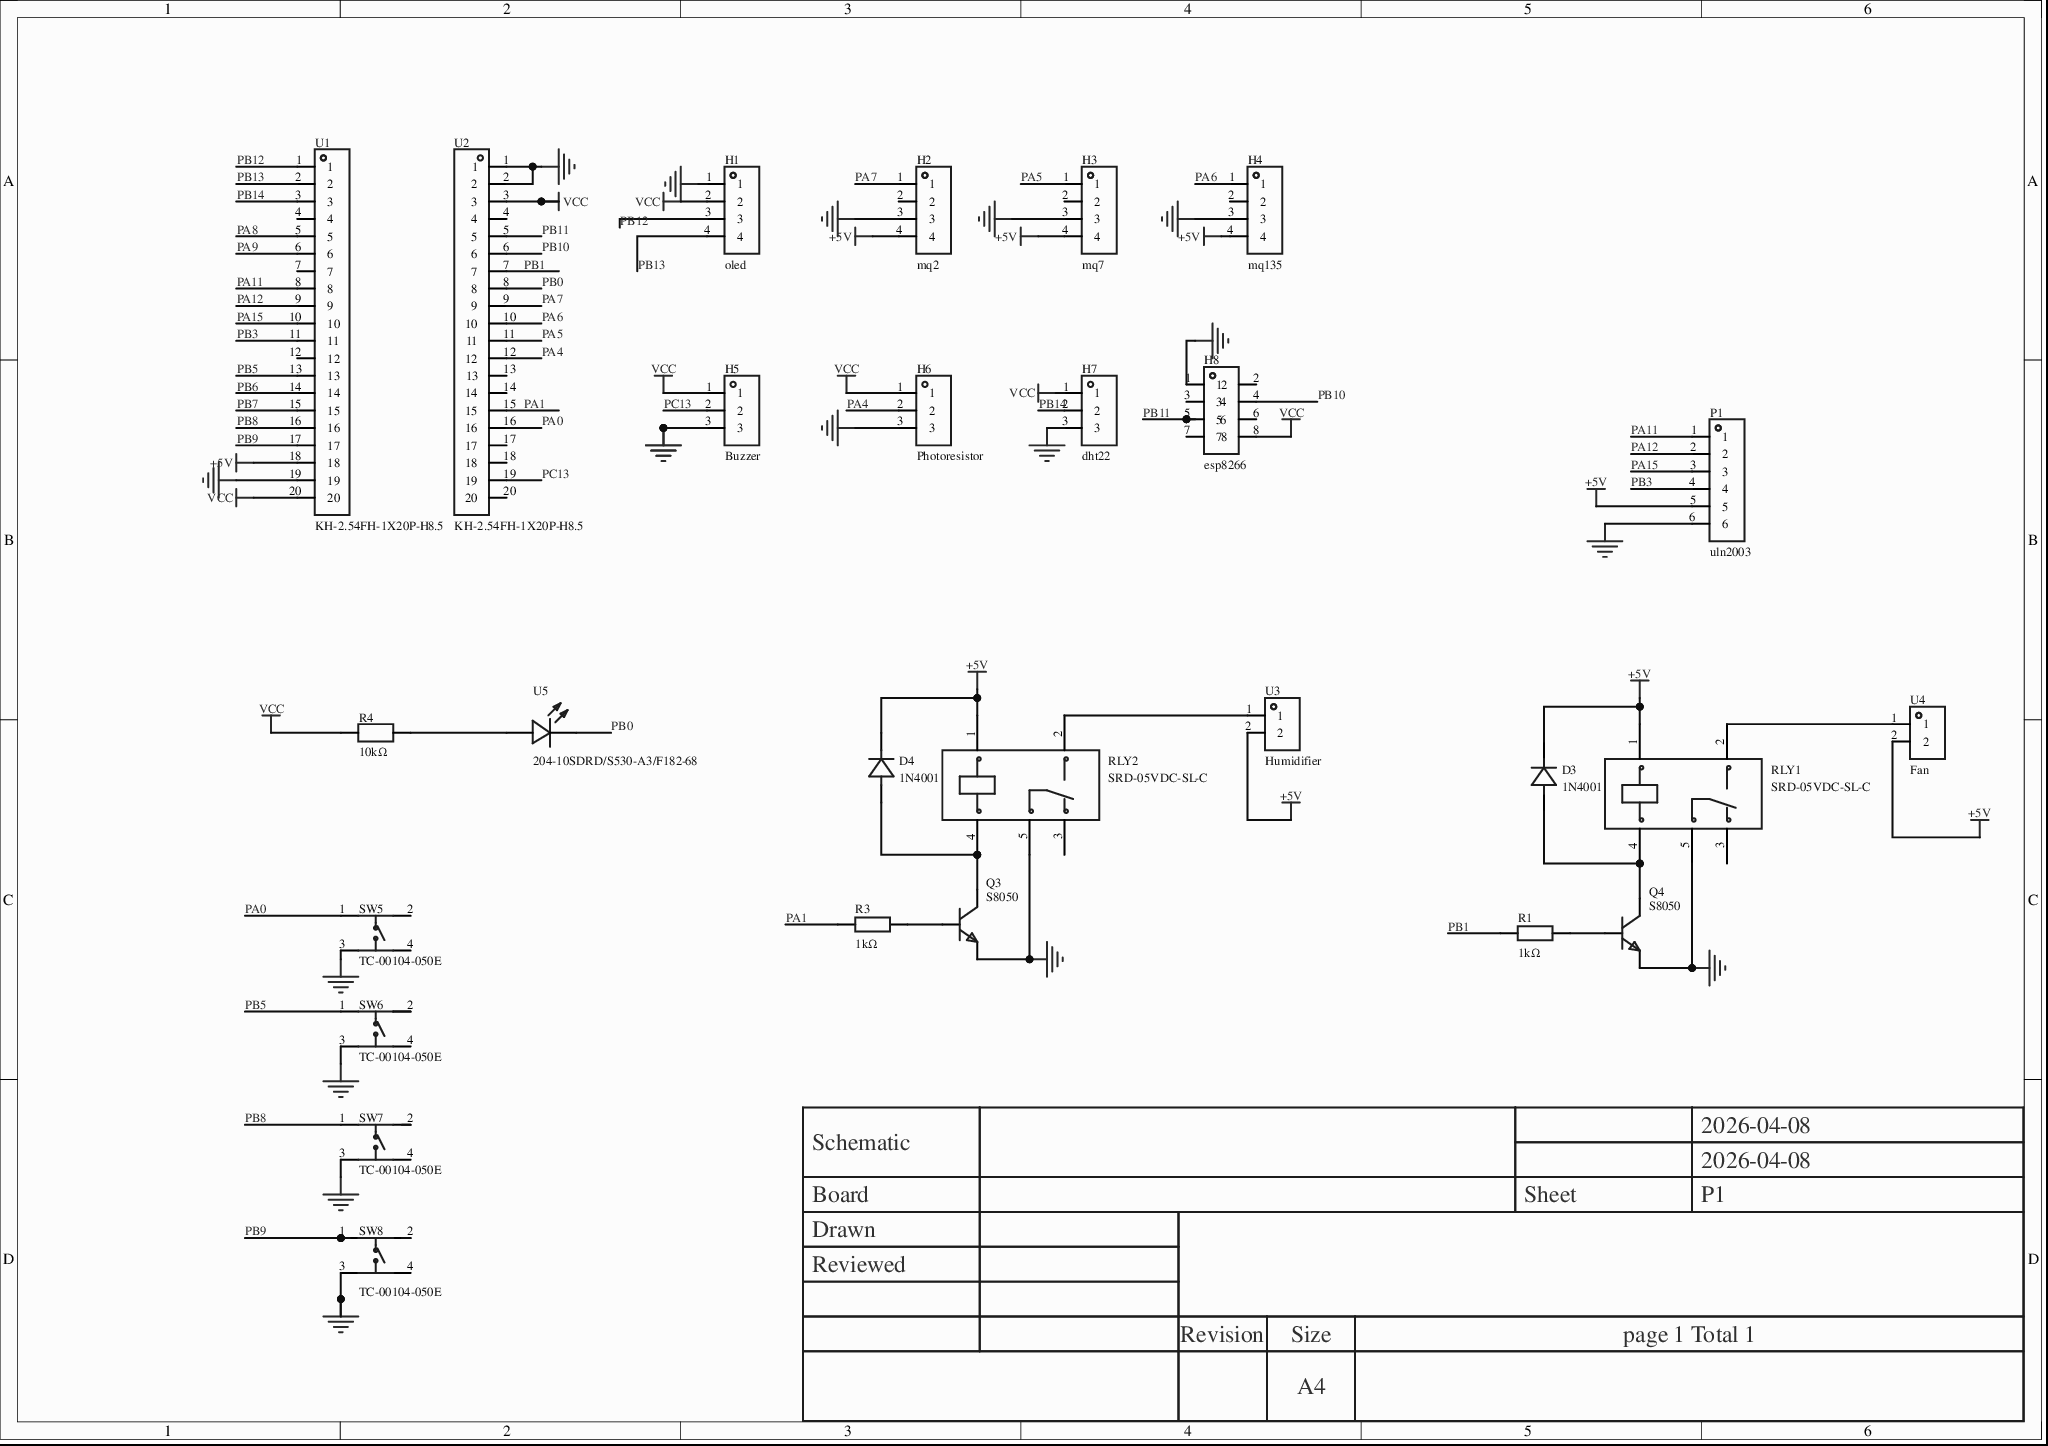
[diagram p0: MISC51563-3.schdoc]
# Altium project MISC51563-2.PrjPcb
1 sheet, 27 parts. Net scope: global (net labels, ports and power ports of the same name join across sheets).
Board file: MISC51563.pcbdoc

## Sheet MISC51563-3.schdoc
size 297 x 209 mm; Version: V1.0; @Project Name: MISC51563; @Update Date: 2026-04-22; @Create Date: 2026-04-22; @Board Name: MISC51563; @Create Time: 22:07:17; @Page Count: 1; @Page No: 1; @Schematic Name: MISC51563; @Update Time: 22:07:17; Size: A4

### Parts
D3  1N4001  [DO-41_BD2.4-L4.7-P8.70-D0.9-RD]
D4  1N4001  [DO-41_BD2.4-L4.7-P8.70-D0.9-RD]
H1  oled  [HDR-TH_4P-P2.54-V-F]
H2  mq2  [HDR-TH_4P-P2.54-V-F]
H3  mq7  [HDR-TH_4P-P2.54-V-F]
H4  mq135  [HDR-TH_4P-P2.54-V-F]
H5  Buzzer  [HDR-TH_3P-P2.54-V-F]
H6  Photoresistor  [HDR-TH_3P-P2.54-V-F]
H7  dht22  [HDR-TH_3P-P2.54-V-F]
H8  esp8266  [HDR-TH_8P-P2.54-V-F-R2-C4-S2.54]
P1  uln2003  [HDR-TH_6P-P2.54-V-F]
Q3  S8050  [TO-92-3_L4.5-W3.5-P1.27-L]
Q4  S8050  [TO-92-3_L4.5-W3.5-P1.27-L]
R1  1kΩ  [RES-TH_BD2.5-L6.5-P10.50-D0.6]
R3  1kΩ  [RES-TH_BD2.5-L6.5-P10.50-D0.6]
R4  10kΩ  [RES-TH_BD2.7-L6.2-P10.20-D0.4]
RLY1  SRD-05VDC-SL-C  [RELAY-TH_SRD-XXVDC-XL-C]
RLY2  SRD-05VDC-SL-C  [RELAY-TH_SRD-XXVDC-XL-C]
SW5  TC-00104-050E  [SW-TH_4P-L6.0-W6.0-P4.50-LS6.5]
SW6  TC-00104-050E  [SW-TH_4P-L6.0-W6.0-P4.50-LS6.5]
SW7  TC-00104-050E  [SW-TH_4P-L6.0-W6.0-P4.50-LS6.5]
SW8  TC-00104-050E  [SW-TH_4P-L6.0-W6.0-P4.50-LS6.5]
U1  KH-2.54FH-1X20P-H8.5  [HDR-TH_20P-P2.54-V-F-2]
U2  KH-2.54FH-1X20P-H8.5  [HDR-TH_20P-P2.54-V-F-2]
U3  Humidifier  [HDR-TH_2P-P2.54-V-F]
U4  Fan  [HDR-TH_2P-P2.54-V-F]
U5  204-10SDRD/S530-A3/F182-68  [LED-TH_BD4.0-P2.50-RD]

### Nets
+5V: D3.1(K) D4.1(K) H2.4 H3.4 H4.4 P1.5 RLY1.1 RLY2.1 U1.18 U3.2 U4.2
GND: H1.1 H2.3 H3.3 H4.3 H5.3 H6.3 H7.3 H8.1 P1.6 Q3.1(E) Q4.1(E) RLY1.5 RLY2.5 SW5.3(C) SW6.3(C) SW7.3(C) SW8.3(C) U1.19 U2.1 U2.2
VCC: H1.2 H5.1 H6.1 H7.1 H8.8 R4.1 U1.20 U2.3
PA0: SW5.1(A) U2.16
PA1: R3.1 U2.15
PA4: H6.2 U2.12
PA5: H3.1 U2.11
PA6: H4.1 U2.10
PA7: H2.1 U2.9
PA8: U1.5
PA9: U1.6
PA11: P1.1 U1.8
PA12: P1.2 U1.9
PA15: P1.3 U1.10
PB0: U2.8 U5.1(C)
PB1: R1.1 U2.7
PB3: P1.4 U1.11
PB5: SW6.1(A) U1.13
PB6: U1.14
PB7: U1.15
PB8: SW7.1(A) U1.16
PB9: SW8.1(A) U1.17
PB10: H8.4 U2.6
PB11: H8.5 U2.5
PB12: H1.3 U1.1
PB13: H1.4 U1.2
PB14: H7.2 U1.3
PC13: H5.2 U2.19
NetD3_2: D3.2(A) Q4.3(C) RLY1.4
NetD4_2: D4.2(A) Q3.3(C) RLY2.4
NetQ3_2: Q3.2(B) R3.2
NetQ4_2: Q4.2(B) R1.2
NetR4_2: R4.2 U5.2(A)
NetRLY1_2: RLY1.2 U4.1
NetRLY2_2: RLY2.2 U3.1

Not connected (* = marked no-connect by the designer): H2 2; H3 2; H4 2; H8 2 3 6 7; RLY1 3; RLY2 3; SW5 2(B) 4(D); SW6 2(B) 4(D); SW7 2(B) 4(D); SW8 2(B) 4(D); U1 4 7 12; U2 4 13 14 17 18 20

### Notes on the sheet
- 2026-04-08
- Schematic
- Board
- Sheet
- P1
- Drawn
- Reviewed
- Revision
- Size
- A4
- page 1 Total 1

### Library data of the parts
D3 D4 = 1N4001_C5359862: Diode configuration: independent; forward voltage drop (Vf): 1V@1A; DC reverse withstand voltage (Vr): 50V; rectified current: 1A;; Manufacturer: LGE(鲁光); AddInBom: yes; Reverse Leakage Current (Ir): 5uA@50V; Operating Junction Temperature Range: -65℃~+150℃; ModelId: 6de1e9b71a0d4751b4e9df530304c1a30819f05c4eef4c71ace90d822a990e87; ModelName: DO-41_D2.4-L4.7-P8.70; ModelTransform: 373.9,94.4,232.29,0,0,0,0,0,-140; Device: 1N4001_C5359862; Symbol: 1N4001_C5359862; FootprintName: DO-41_BD2.4-L4.7-P8.70-D0.9-RD; LCSC Part Name: 50V 1A; SupplierPart: C5359862; ManufacturerPart: 1N4001; Supplier Footprint: DO-41; JLCPCB Part Class: Extended Part; Datasheet: example.com/datasheet/1N4001/6175385.html; Supplier: LCSC; ConvertToPcb: yes; Diode Configuration: Independent; Voltage - Forward(Vf@If): 1V@1A; Voltage - DC Reverse(Vr): 50V; Current - Rectified: 1A; Non-Repetitive Peak Forward Surge Current: -
H1-H4 = 2.54-1*4P母: Socket structure: 1x4P; pitch: 2.54mm; row spacing: -; round/square hole: square hole; mounting: through-hole; rows: single row; total positions: 4P; rated current: 3A; rated voltage: -; hole direction: top; plastic height: -; contact material: bronze; contact plating: -; operating temperature: -40℃~+105℃;; Manufacturer: BOOMELE(博穆精密); Device: 2.54-1*4P female; AddInBom: yes; ModelId: d187812051054f85879fcaa51a310d8e0819f05c4eef4c71ace90d822a990e87; ModelTransform: 419.6842,98.464,0,0,0,0,0,0,-118.11; Symbol: 2.54-1*4P female; FootprintName: HDR-TH_4P-P2.54-V-F; LCSC Part Name: 间距:2.54mm 1x4P 直插; SupplierPart: C2718488; Supplier Footprint: 插件,P=2.54mm; JLCPCB Part Class: Extended Part; Datasheet: example.com/datasheet/2.54-1*4P%25E6%25AF%258D/2834502.html; Supplier: LCSC; ConvertToPcb: yes; Holes Structure: 1x4P; Pitch: 2.54mm; Row Spacing: -; Circular Hole / Square Hole: Square hole; Mounting Type: Through-hole; Number of Rows: Single row; Number of Positions: 4P; Current Rating: 3A; Voltage Rating (Max): -; Holes Direction: Top; Insulation Height: -; Contact Material: Bronze; Contact Plating: -; Operating Temperature: -40℃~+105℃; ModelName: HDR-TH_4P-P2.54-V-F
  H1: Manufacturer Part: oled
  H2: Manufacturer Part: mq2
  H3: Manufacturer Part: mq7
  H4: Manufacturer Part: mq135
H5 = PM254V-11-03-H85: Socket structure: 1x3P; pitch: 2.54mm; row spacing: -; round/square hole: square hole; mounting: through-hole; rows: single row; total positions: 3P; rated current: 3A; hole direction: top; plastic height: 8.5mm; contact material: brass; contact plating: -; operating temperature: -40℃~+105℃;; Manufacturer Part: 蜂鸣器; Manufacturer: XFCN(兴飞); AddInBom: yes; ModelId: f3b3cc5aae9641bf9e56fc160cef875b0819f05c4eef4c71ace90d822a990e87; ModelName: HDR2.54-F-LI-1X3P; ModelTransform: 299.9994,100,0,0,0,0,0,0,-118.11; Device: PM254V-11-03-H85; Symbol: PM254V-11-03-H85; FootprintName: HDR-TH_3P-P2.54-V-F; LCSC Part Name: 1x3P 间距:2.54mm 直插; SupplierPart: C541850; Supplier Footprint: 插件,P=2.54mm; JLCPCB Part Class: Extended Part; Datasheet: example.com/datasheet/PM254V-11-03-H85/562471.html; Supplier: LCSC; ConvertToPcb: yes; Holes Structure: 1x3P; Pitch: 2.54mm; Row Spacing: -; Circular Hole / Square Hole: Square hole; Mounting Type: Through-hole; Number of Rows: Single row; Number of Positions: 3P; Current Rating: 3A; Holes Direction: Top; Insulation Height: 8.5mm; Contact Material: Brass; Contact Plating: -; Operating Temperature: -40℃~+105℃
H6 = PM254V-11-03-H85: Socket structure: 1x3P; pitch: 2.54mm; row spacing: -; round/square hole: square hole; mounting: through-hole; rows: single row; total positions: 3P; rated current: 3A; hole direction: top; plastic height: 8.5mm; contact material: brass; contact plating: -; operating temperature: -40℃~+105℃;; Manufacturer Part: 光敏; Manufacturer: XFCN(兴飞); AddInBom: yes; ModelId: f3b3cc5aae9641bf9e56fc160cef875b0819f05c4eef4c71ace90d822a990e87; ModelName: HDR2.54-F-LI-1X3P; ModelTransform: 299.9994,100,0,0,0,0,0,0,-118.11; Device: PM254V-11-03-H85; Symbol: PM254V-11-03-H85; FootprintName: HDR-TH_3P-P2.54-V-F; LCSC Part Name: 1x3P 间距:2.54mm 直插; SupplierPart: C541850; Supplier Footprint: 插件,P=2.54mm; JLCPCB Part Class: Extended Part; Datasheet: example.com/datasheet/PM254V-11-03-H85/562471.html; Supplier: LCSC; ConvertToPcb: yes; Holes Structure: 1x3P; Pitch: 2.54mm; Row Spacing: -; Circular Hole / Square Hole: Square hole; Mounting Type: Through-hole; Number of Rows: Single row; Number of Positions: 3P; Current Rating: 3A; Holes Direction: Top; Insulation Height: 8.5mm; Contact Material: Brass; Contact Plating: -; Operating Temperature: -40℃~+105℃
H7 = PM254V-11-03-H85: Socket structure: 1x3P; pitch: 2.54mm; row spacing: -; round/square hole: square hole; mounting: through-hole; rows: single row; total positions: 3P; rated current: 3A; hole direction: top; plastic height: 8.5mm; contact material: brass; contact plating: -; operating temperature: -40℃~+105℃;; Manufacturer: XFCN(兴飞); AddInBom: yes; ModelId: f3b3cc5aae9641bf9e56fc160cef875b0819f05c4eef4c71ace90d822a990e87; ModelName: HDR2.54-F-LI-1X3P; ModelTransform: 299.9994,100,0,0,0,0,0,0,-118.11; Device: PM254V-11-03-H85; Symbol: PM254V-11-03-H85; Manufacturer Part: dht22; FootprintName: HDR-TH_3P-P2.54-V-F; LCSC Part Name: 1x3P 间距:2.54mm 直插; SupplierPart: C541850; Supplier Footprint: 插件,P=2.54mm; JLCPCB Part Class: Extended Part; Datasheet: example.com/datasheet/PM254V-11-03-H85/562471.html; Supplier: LCSC; ConvertToPcb: yes; Holes Structure: 1x3P; Pitch: 2.54mm; Row Spacing: -; Circular Hole / Square Hole: Square hole; Mounting Type: Through-hole; Number of Rows: Single row; Number of Positions: 3P; Current Rating: 3A; Holes Direction: Top; Insulation Height: 8.5mm; Contact Material: Brass; Contact Plating: -; Operating Temperature: -40℃~+105℃
H8 = PM254V-12-08-H85: Socket structure: 2x4P; pitch: 2.54mm; row spacing: 2.54mm; round/square hole: square hole; mounting: through-hole; rows: double row; total positions: 8P; rated current: 3A; rated voltage: 250V; hole direction: top; plastic height: 8.5mm; operating temperature: -40℃~+105℃;; Manufacturer: XFCN(兴飞); Symbol: PM254V-12-08-H85_C2834799; AddInBom: yes; ModelId: 52f9c7b3691648c0a1959c61eae445900819f05c4eef4c71ace90d822a990e87; ModelName: HDR-TH_8P-P2.54-F-LI-2X4P; ModelTransform: 415.7472,196.85,0,0,0,0,0,0,-118.11; Device: PM254V-12-08-H85; Manufacturer Part: esp8266; FootprintName: HDR-TH_8P-P2.54-V-F-R2-C4-S2.54; LCSC Part Name: 间距:2.54mm 2x4P 直插; SupplierPart: C2834799; Supplier Footprint: 插件,P=2.54mm; JLCPCB Part Class: Extended Part; Datasheet: example.com/datasheet/PM254V-12-08-H85/2997439.html; Supplier: LCSC; ConvertToPcb: yes; Holes Structure: 2x4P; Pitch: 2.54mm; Row Spacing: 2.54mm; Circular Hole / Square Hole: Square hole; Mounting Type: Through-hole; Number of Rows: Double row; Number of Positions: 8P; Current Rating: 3A; Voltage Rating (Max): 250V; Holes Direction: Top; Insulation Height: 8.5mm; Operating Temperature: -40℃~+105℃
P1 = 2.54-1*6P母: Socket structure: 1x6P; pitch: 2.54mm; row spacing: -; round/square hole: square hole; mounting: through-hole; rows: single row; total positions: 6P; rated current: 3A; rated voltage: -; hole direction: top; plastic height: -; contact material: brass; contact plating: -; operating temperature: -40℃~+105℃;; Manufacturer: BOOMELE(博穆精密); Device: 2.54-1*6P female; Symbol: Header-Female-2.54_1x6; AddInBom: yes; PIN Length: 3.3mm; ModelId: 0f5bcf94dcda47d085f24cdca1696fe90819f05c4eef4c71ace90d822a990e87; ModelTransform: 619.684,94.488,0,0,0,0,0,0,-125.984; Manufacturer Part: uln2003; FootprintName: HDR-TH_6P-P2.54-V-F; LCSC Part Name: 1x6P 间距:2.54mm 直插; SupplierPart: C40877; Supplier Footprint: 插件,P=2.54mm; JLCPCB Part Class: Extended Part; Datasheet: example.com/datasheet/2.54-1*6P%25E6%25AF%258D/41861.html; Supplier: LCSC; ConvertToPcb: yes; Holes Structure: 1x6P; Pitch: 2.54mm; Row Spacing: -; Circular Hole / Square Hole: Square hole; Mounting Type: Through-hole; Number of Rows: Single row; Number of Positions: 6P; Current Rating: 3A; Voltage Rating (Max): -; Holes Direction: Top; Insulation Height: -; Contact Material: Brass; Contact Plating: -; Operating Temperature: -40℃~+105℃; Supplementary Features: -; ModelName: HDR-TH_6P-P2.54-V-F
Q3 Q4 = S8050_C2931492: Transistor type: NPN; collector current (Ic): 500mA; collector-emitter breakdown voltage (Vceo): 25V; power dissipation (Pd): 625mW; DC current gain (hFE): 160@50mA,1V;; Manufacturer: JSMSEMI(杰盛微); AddInBom: yes; Transition frequency(fT): 150MHz; Current - Collector Cutoff: 100nA; Vce Saturation(VCE(sat)): 600mV@500mA,50mA; Emitter-Base Voltage(Vebo): 5V; ModelId: 45fa6cddef3743c6aacf8db740a3bc4c0819f05c4eef4c71ace90d822a990e87; ModelTransform: 177.165,137.795,0,0,0,0,0,29.528,-98.425; Device: S8050_C2931492; Symbol: S8050_C2931492; FootprintName: TO-92-3_L4.5-W3.5-P1.27-L; LCSC Part Name: NPN 电流:500mA 电压:25V; SupplierPart: C2931492; ManufacturerPart: S8050; Supplier Footprint: TO-92; JLCPCB Part Class: Extended Part; Datasheet: example.com/datasheet/S8050/3272796.html; Supplier: LCSC; ConvertToPcb: yes; type: NPN; Current - Collector(Ic): 500mA; Collector - Emitter Voltage VCEO: 25V; Pd - Power Dissipation: 625mW; DC Current Gain: 160@50mA,1V; ModelName: TO-92-3_L4.5-W3.5-P1.27-L
R1 R3 = MFR0W4F1001A50: Resistor type: metal film resistor; resistance: 1kΩ; tolerance: ±1%; power: 250mW; temperature coefficient: ±50ppm/℃;; Manufacturer: UNI-ROYAL(厚声); AddInBom: yes; Voltage-Supply(Max): 250V; ModelId: 8e6c7ee8323443d1ab8f0504b6353c8c0819f05c4eef4c71ace90d822a990e87; ModelName: RES-TH_D2.3-L6.5-P10.50; ModelTransform: 431.1015,91.3384,0,0,0,0,0.197,0,-137.795; Device: MFR0W4F1001A50; Symbol: MFR0W4F1001A50; FootprintName: RES-TH_BD2.5-L6.5-P10.50-D0.6; LCSC Part Name: 1kΩ ±1% 250mW 金属膜电阻 铜脚，圆柱状直插; SupplierPart: C57435; ManufacturerPart: MFR0W4F1001A50; Supplier Footprint: 插件,D2.2xL6.5mm; JLCPCB Part Class: Extended Part; Datasheet: example.com/upload/public/pdf/source/20191012/C436293_8820AA14BC71FA35E551C06C441482A0.pdf; Supplier: LCSC; ConvertToPcb: yes; Type: Metal film resistor; Value: 1kΩ; Tolerance: ±1%; Power(Watts): 250mW; Temperature Coefficient: ±50ppm/℃
R4 = MF1/4W-10K±1%-ST52: Resistor type: metal film resistor; resistance: 10kΩ; tolerance: ±1%; power: 250mW; temperature coefficient: ±100ppm/℃;; Manufacturer: VO(翔胜); AddInBom: yes; Voltage-Supply(Max): 250V; ModelId: f91fbe0e2e6f409498f09f811e4616fe0819f05c4eef4c71ace90d822a990e87; ModelTransform: 417.322,106.221,0,0,0,0,0,0,-196.85; Device: MF1/4W-10K±1%-ST52; Symbol: MF1/4W-10K±1%-ST52; FootprintName: RES-TH_BD2.7-L6.2-P10.20-D0.4; LCSC Part Name: 金属膜电阻 10kΩ ±1% 250mW; SupplierPart: C2903232; ManufacturerPart: MF1/4W-10K±1%-ST52; Supplier Footprint: 插件,D2.7xL6.2mm; JLCPCB Part Class: Extended Part; Datasheet: example.com/datasheet/MF1%252F4W-10K%25C2%25B11%2525-ST52/3158983.html; Supplier: LCSC; ConvertToPcb: yes; Type: Metal film resistor; Value: 10kΩ; Tolerance: ±1%; Power(Watts): 250mW; Temperature Coefficient: ±100ppm/℃; Operating Temperature: -55℃~+155℃; ModelName: RES-TH_BD2.7-L6.2-P10.20-D0.4
RLY1 RLY2 = SRD-05VDC-SL-C: Coil voltage: 5V; contact form: changeover 1C (SPDT); contact rating (resistive load): -; max switching voltage: 250V@AC; max switching current: 15A;; Manufacturer: 松乐; 3D Model: d0eda9b8bf8746d18ae810ab88dc78e70819f05c4eef4c71ace90d822a990e87; 3D Model Transform: 755.904,622.4397,0,0,0,0,34.882,0,-118.11; Contact Form: Changeover: 1C (SPDT); Coil Rated Power: 360mW; Coil Type: Non-polar, single coil; Coil Resistance: 70Ω; Contact Resistance: 100mΩ; Operate Time: 10ms; AddInBom: yes; ModelName: RELAY-TH_L19.2-W15.6-H15.8; Device: SRD-05VDC-SL-C; Symbol: SRD-05VDC-SL-C; LCSC Part Name: 蓝色 单组转换型继电器; Supplier Part: C35449; Manufacturer Part: SRD-05VDC-SL-C; Supplier Footprint: 插件,15.6x19.2mm; JLCPCB Part Class: Extended Part; Datasheet: example.com/datasheet/SRD-05VDC-SL-C/36422.html; Supplier: LCSC; Coil Voltage: 5V; Number of Pins: 5; Contact Rating: -; Switching Voltage(Max): 250V@AC; Switching Current(Max): 15A; Release Time: 10ms; FootprintName: RELAY-TH_SRD-XXVDC-XL-C; ConvertToPcb: yes
SW5-SW8 = TC-00104-050E: Circuit structure: SPST; button shape: round button; actuation force: 2.5N; mounting: through-hole; switch length: 6mm; switch width: 6mm; switch height: 5mm; bracket: without bracket; lamp: none; operating life: -;; Manufacturer: HOOYA(皓宇电子); AddInBom: yes; Actuator/Cap Color: Black; ModelId: 20eee248bc684ccd8cbdbb1d0d91ec6f0819f05c4eef4c71ace90d822a990e87; ModelName: SW-TH_4P-L6.0-W6.0-H5.0-LS6.5-P4.50; ModelTransform: 236.22,323.03,0,90,0,0,0,0,-137.795; Device: TC-00104-050E; Symbol: TC-00104-050E; FootprintName: SW-TH_4P-L6.0-W6.0-P4.50-LS6.5; LCSC Part Name: 6mm*6mm*5mm; SupplierPart: C2939600; ManufacturerPart: TC-00104-050E; Supplier Footprint: 插件,6x6mm; JLCPCB Part Class: Extended Part; Datasheet: example.com/datasheet/TC-00104-050E/3300585.html; Supplier: LCSC; ConvertToPcb: yes; Circuit: SPST; Actuator Style: Round button; Operating Force: 2.5N; Mounting Type: Through-hole; Length: 6mm; Width: 6mm; Switch Height: 5mm; with Bracket: Without bracket; With Lamp: None; IP Rating: -; Termination Style: PC pins; Life: -
U1 U2 = KH-2.54FH-1X20P-H8.5: Socket structure: 1x20P; pitch: 2.54mm; row spacing: -; round/square hole: square hole; mounting: through-hole; rows: single row; total positions: 20P; rated current: 3A; rated voltage: -; hole direction: top; plastic height: 8.5mm; operating temperature: -40℃~+105℃;; Manufacturer: kinghelm(金航标); AddInBom: yes; ModelId: 48d3332f1f604cb48783c9ca75931f3b0819f05c4eef4c71ace90d822a990e87; ModelTransform: 1999.996,98.8187,0,0,0,0,0,0,-106.299; Device: KH-2.54FH-1X20P-H8.5; Symbol: KH-2.54FH-1X20P-H8.5; FootprintName: HDR-TH_20P-P2.54-V-F-2; LCSC Part Name: 间距:2.54mm 1x20P 直插; SupplierPart: C2905423; ManufacturerPart: KH-2.54FH-1X20P-H8.5; Supplier Footprint: 插件,P=2.54mm; JLCPCB Part Class: Extended Part; Datasheet: example.com/datasheet/KH-2.54FH-1X20P-H8.5/3175197.html; Supplier: LCSC; ConvertToPcb: yes; Holes Structure: 1x20P; Pitch: 2.54mm; Row Spacing: -; Circular Hole / Square Hole: Square hole; Mounting Type: Through-hole; Number of Rows: Single row; Number of Positions: 20P; Current Rating: 3A; Voltage Rating (Max): -; Holes Direction: Top; Insulation Height: 8.5mm; Operating Temperature: -40℃~+105℃; ModelName: HDR-TH_20P-P2.54-V-F-2
U3 = ZX-PM2.54-1-2PY: Socket structure: 1x2P; pitch: 2.54mm; row spacing: -; round/square hole: square hole; mounting: through-hole; rows: single row; total positions: 2P; rated current: 3A; rated voltage: -; hole direction: top; plastic height: 8.5mm; contact material: brass; contact plating: gold; operating temperature: -40℃~+105℃;; Manufacturer Part: 加湿器; Manufacturer: Megastar(兆星); AddInBom: yes; PIN Length: 3.2mm; ModelId: a9450ef445564560a104363b9aacde4e0819f05c4eef4c71ace90d822a990e87; ModelName: HDR-TH_2P-P2.54-F-LI-1X2P; ModelTransform: 215.7476,98.425,0,0,0,0,0,0,-129.921; Device: ZX-PM2.54-1-2PY; Symbol: ZX-PM2.54-1-2PY; FootprintName: HDR-TH_2P-P2.54-V-F; LCSC Part Name: 1x2P 间距:2.54mm 直插; SupplierPart: C7499322; Supplier Footprint: 插件,P=2.54mm; JLCPCB Part Class: Extended Part; Datasheet: example.com/datasheet/ZX-PM2.54-1-2PY/8573983.html; Supplier: LCSC; ConvertToPcb: yes; Holes Structure: 1x2P; Pitch: 2.54mm; Row Spacing: -; Circular Hole / Square Hole: Square hole; Mounting Type: Through-hole; Number of Rows: Single row; Number of Positions: 2P; Current Rating: 3A; Voltage Rating (Max): -; Holes Direction: Top; Insulation Height: 8.5mm; Contact Material: Brass; Contact Plating: Gold; Operating Temperature: -40℃~+105℃
U4 = ZX-PM2.54-1-2PY: Socket structure: 1x2P; pitch: 2.54mm; row spacing: -; round/square hole: square hole; mounting: through-hole; rows: single row; total positions: 2P; rated current: 3A; rated voltage: -; hole direction: top; plastic height: 8.5mm; contact material: brass; contact plating: gold; operating temperature: -40℃~+105℃;; Manufacturer Part: 风扇; Manufacturer: Megastar(兆星); AddInBom: yes; PIN Length: 3.2mm; ModelId: a9450ef445564560a104363b9aacde4e0819f05c4eef4c71ace90d822a990e87; ModelName: HDR-TH_2P-P2.54-F-LI-1X2P; ModelTransform: 215.7476,98.425,0,0,0,0,0,0,-129.921; Device: ZX-PM2.54-1-2PY; Symbol: ZX-PM2.54-1-2PY; FootprintName: HDR-TH_2P-P2.54-V-F; LCSC Part Name: 1x2P 间距:2.54mm 直插; SupplierPart: C7499322; Supplier Footprint: 插件,P=2.54mm; JLCPCB Part Class: Extended Part; Datasheet: example.com/datasheet/ZX-PM2.54-1-2PY/8573983.html; Supplier: LCSC; ConvertToPcb: yes; Holes Structure: 1x2P; Pitch: 2.54mm; Row Spacing: -; Circular Hole / Square Hole: Square hole; Mounting Type: Through-hole; Number of Rows: Single row; Number of Positions: 2P; Current Rating: 3A; Voltage Rating (Max): -; Holes Direction: Top; Insulation Height: 8.5mm; Contact Material: Brass; Contact Plating: Gold; Operating Temperature: -40℃~+105℃
U5 = 204-10SDRD/S530-A3/F182-68: -; Manufacturer: EVERLIGHT(亿光); AddInBom: yes; ModelId: 8e04cf257f6f425a9619e557bdb7ad570819f05c4eef4c71ace90d822a990e87; ModelName: LED-TH_BD4.0-P2.50-H6.0-RD; ModelTransform: 169.291,180.65972,0,0,0,0,5.08,-0.001,-196.85; Device: 204-10SDRD/S530-A3/F182-68; Symbol: 204-10SDRD/S530-A3/F182-68; FootprintName: LED-TH_BD4.0-P2.50-RD; LCSC Part Name: 204-10SDRD/S530-A3/F182-68; SupplierPart: C473831; ManufacturerPart: 204-10SDRD/S530-A3/F182-68; Supplier Footprint: 插件; JLCPCB Part Class: Extended Part; Supplier: LCSC; ConvertToPcb: yes